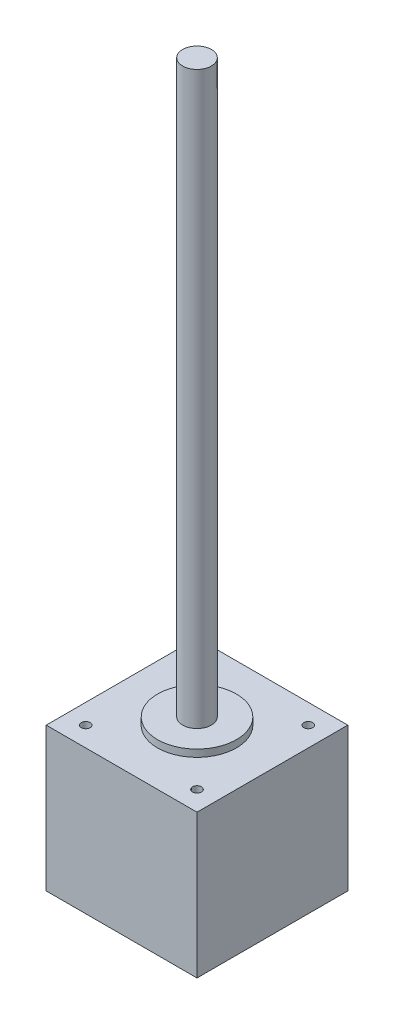
from build123d import *

# Parameters (mm, degrees)
SKETCH1_W             = 42
SKETCH1_H             = 42
BOSS_EXTRUDE1_DEPTH   = 40
SKETCH2_R             = 11
BOSS_EXTRUDE2_DEPTH   = 2
SKETCH3_R             = 4
BOSS_EXTRUDE3_DEPTH   = 159
SKETCH4_R             = 0.75
CUT_EXTRUDE1_DEPTH    = 5
M3_TAPPED_HOLE1_D     = 2.5
M3_TAPPED_HOLE1_DEPTH = 7.5
M3_TAPPED_HOLE1_TIP   = 0.751075774


with BuildPart() as part:
    # Sketch1 → Boss-Extrude1 (new body)
    with BuildSketch(Plane(origin=(0, 0, 0), x_dir=(1, 0, 0), z_dir=(0, 1, 0))):
        Rectangle(SKETCH1_W, SKETCH1_H)
    extrude(amount=BOSS_EXTRUDE1_DEPTH)

    # Sketch2 → Boss-Extrude2 (add)
    with BuildSketch(Plane(origin=(0, 40, 0), x_dir=(1, 0, 0), z_dir=(0, 1, 0))):
        with Locations(Location((0, 0, 0), (0, 0, 270))):
            Circle(SKETCH2_R)
    extrude(amount=BOSS_EXTRUDE2_DEPTH)

    # Sketch3 → Boss-Extrude3 (add)
    with BuildSketch(Plane(origin=(0, 42, 0), x_dir=(1, 0, 0), z_dir=(0, 1, 0))):
        with Locations(Location((0, 0, 0), (0, 0, 90))):
            Circle(SKETCH3_R)
    extrude(amount=BOSS_EXTRUDE3_DEPTH)

    # Sketch4 → Cut-Extrude1 (cut)
    with BuildSketch(Plane(origin=(0, 40, 0), x_dir=(1, 0, 0), z_dir=(0, 1, 0))):
        with Locations(Location((-15.5, 15.5, 0), (0, 0, 270))):
            Circle(SKETCH4_R)
        with Locations(Location((15.5, 15.5, 0), (0, 0, 270))):
            Circle(SKETCH4_R)
        with Locations(Location((15.5, -15.5, 0), (0, 0, 270))):
            Circle(SKETCH4_R)
        with Locations(Location((-15.5, -15.5, 0), (0, 0, 270))):
            Circle(SKETCH4_R)
    extrude(amount=-CUT_EXTRUDE1_DEPTH, mode=Mode.SUBTRACT)

    # M3 Tapped Hole1
    with Locations(Plane(origin=(0, 40, 0), x_dir=(1, 0, 0), z_dir=(0, 1, 0))):
        with Locations((-15.5, 15.5), (15.5, -15.5), (-15.5, -15.5), (15.5, 15.5)):
            Hole(M3_TAPPED_HOLE1_D / 2, depth=M3_TAPPED_HOLE1_DEPTH)
            with Locations((0, 0, -(M3_TAPPED_HOLE1_DEPTH + M3_TAPPED_HOLE1_TIP / 2))):  # 118° drill point
                Cone(0, M3_TAPPED_HOLE1_D / 2, M3_TAPPED_HOLE1_TIP, mode=Mode.SUBTRACT)


solid = part.part
